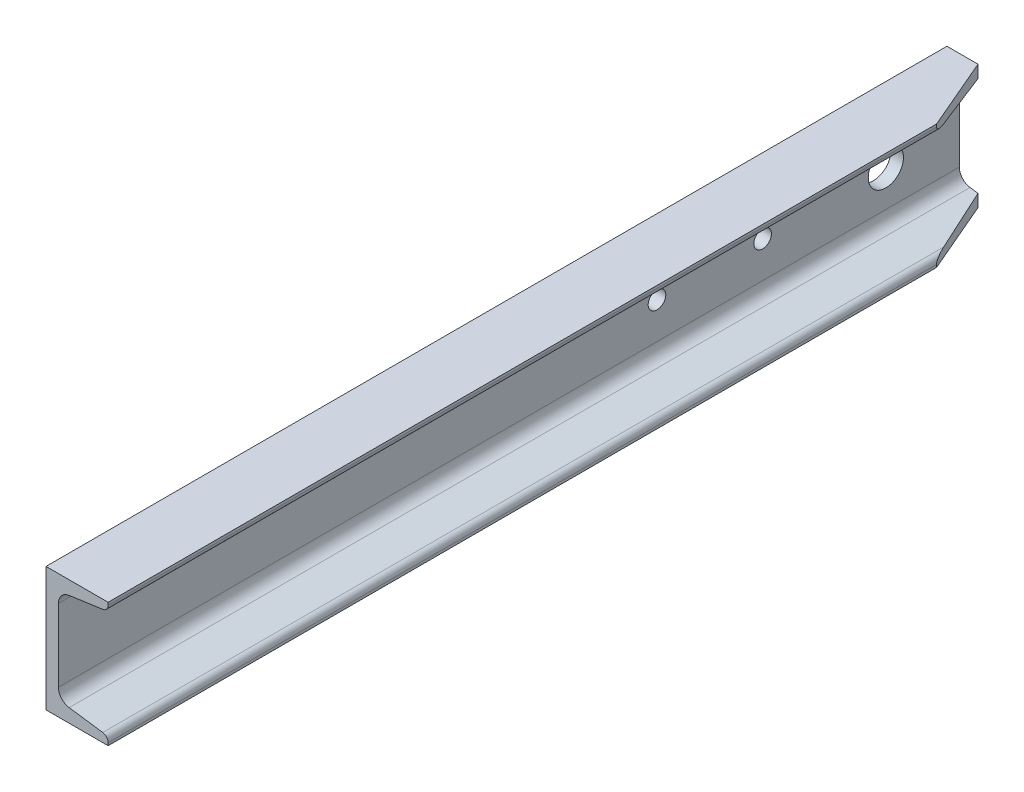
SolidWorks part; units mm, degrees
material "1023 Carbon Steel Plate (SS)"
ref_plane "Front Plane" through (0, 0, 0) normal (0, 0, 1) x (1, 0, 0)
ref_plane "Top Plane" through (0, 0, 0) normal (0, 1, 0) x (1, 0, 0)
ref_plane "Right Plane" through (0, 0, 0) normal (1, 0, 0) x (0, 0, -1)
sketch "Sketch1" plane through (0, 0, 0) normal (0, 0, 1) x (1, 0, 0)
  line L0 (0, 0) -> (-30, 0)
  line L1 (-30, 0) -> (-30, -60)
  line L2 (-30, -60) -> (0, -60)
  line L3 (0, -60) -> (0, -58.716)
  line L4 (-2.5825, -55.7452) -> (-18.835, -53.461)
  line L5 (-24, -47.5194) -> (-24, -12.4806)
  line L6 (-18.835, -6.539) -> (-2.5825, -4.2548)
  line L7 (0, -1.284) -> (0, 0)
  line L8 (-15, -54) -> (-15, -60) construction
  arc A0 (-24, -12.4806) -> (-18.835, -6.539) centre (-18, -12.4806) cw
  arc A1 (-18.835, -53.461) -> (-24, -47.5194) centre (-18, -47.5194) cw
  arc A2 (0, -58.716) -> (-2.5825, -55.7452) centre (-3, -58.716) ccw
  arc A3 (0, -1.284) -> (-2.5825, -4.2548) centre (-3, -1.284) cw
  dimension "D7" = 6
  dimension "D8" = 3
  dimension "D1" = 60
  dimension "D2" = 30
  dimension "D3" = 6
  dimension "D4" = 15
  dimension "D5" = 6
  dimension "D6" = 8
extrude "Boss-Extrude1" add sketch "Sketch1" along normal blind 435 contours A3 L6 A0 L5 A1 L4 A2 L3 L2 L1 L0 L7
sketch "Sketch2" plane through (-30, 0, 0) normal (-1, 0, 0) x (0, 0, 1)
  line L0 (435, 0) -> (435, -60) construction
  circle A0 centre (35.5, -30) radius 8.5
  dimension "D1" = 399.5
  dimension "D2" = 17
extrude "Cut-Extrude1" cut sketch "Sketch2" against normal blind 435
sketch "Sketch3" plane through (0, 0, 0) normal (0, 1, 0) x (1, 0, 0)
  line L0 (-15, 0) -> (0, 0)
  line L2 (0, 0) -> (0, -35)
  line L3 (0, -435) -> (0, 0) construction
  line L4 (0, -35) -> (-15, 0)
  dimension "D1" = 35
  dimension "D2" = 15
extrude "Cut-Extrude2" cut sketch "Sketch3" against normal blind 435
sketch "Sketch4" plane through (-30, 0, 0) normal (-1, 0, 0) x (0, 0, 1)
  line L0 (0, 0) -> (0, -60) construction
  circle A0 centre (95, -30) radius 4.25
  circle A1 centre (146, -30) radius 4.25
  point P8 (0, -30)
  dimension "D3" = 8.5
  dimension "D1" = 95
  dimension "D2" = 51
extrude "Cut-Extrude3" cut sketch "Sketch4" against normal blind 435
